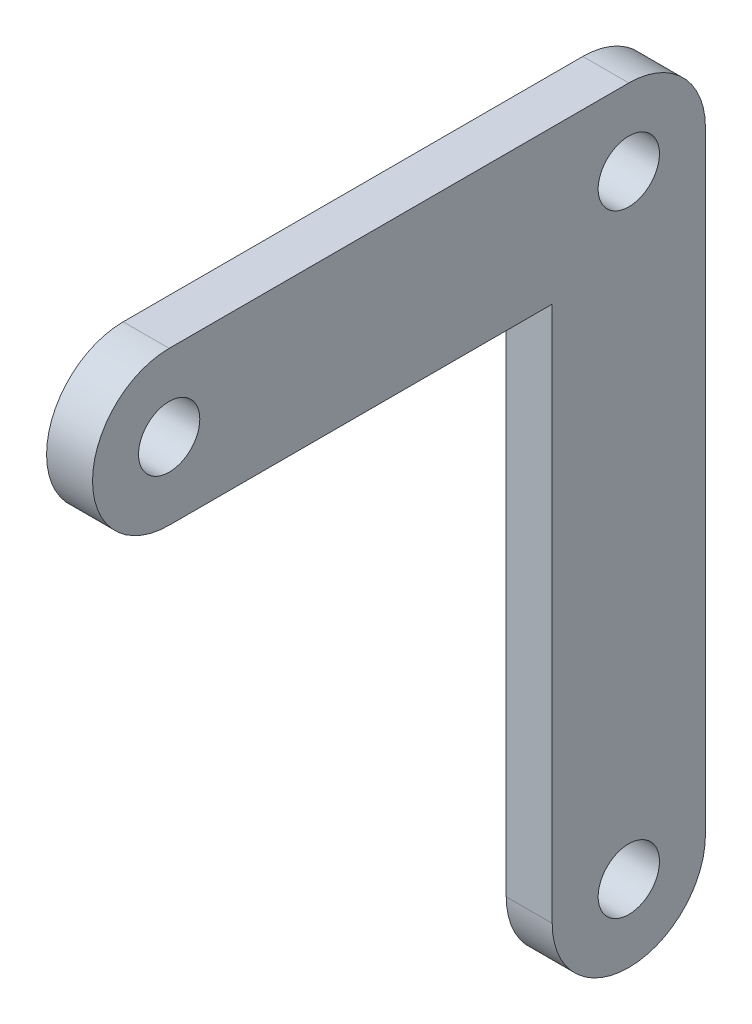
SolidWorks part; units mm, degrees
material "AISI 1045 Steel, cold drawn"
ref_plane "Front Plane" through (0, 0, 0) normal (0, 0, 1) x (1, 0, 0)
ref_plane "Top Plane" through (0, 0, 0) normal (0, 1, 0) x (1, 0, 0)
ref_plane "Right Plane" through (0, 0, 0) normal (1, 0, 0) x (0, 0, -1)
sketch "Sketch1" plane through (0, 0, 0) normal (1, 0, 0) x (0, 0, -1)
  line L0 (0, 0) -> (60, 0) construction
  line L1 (60, 0) -> (60, -80) construction
  line L2 (0, 0) -> (60, 0) construction
  line L3 (0, 10) -> (60, 10)
  line L4 (0, -10) -> (60, -10)
  line L5 (60, 0) -> (60, -80) construction
  line L6 (70, 0) -> (70, -80)
  line L7 (50, 0) -> (50, -80)
  line L8 (55, 0) -> (-55, 0) construction
  arc A0 (0, 10) -> (0, -10) centre (0, 0) ccw
  arc A1 (60, -10) -> (60, 10) centre (60, 0) ccw
  arc A2 (70, 0) -> (50, 0) centre (60, 0) ccw
  arc A3 (50, -80) -> (70, -80) centre (60, -80) ccw
  circle A4 centre (0, 0) radius 4
  circle A5 centre (60, 0) radius 4
  circle A6 centre (60, -80) radius 4
  point P3 (30, 0)
  point P9 (60, -40)
  dimension "D3" = 10
  dimension "D4" = 8
  dimension "D1" = 60
  dimension "D2" = 80
extrude "Boss-Extrude1" add sketch "Sketch1" along normal blind 6 contours A2 L3 A0 L4 L7 A4 | A1 A2 L7 L4 A5 | L7 A3 L6 A1 L4 A6
